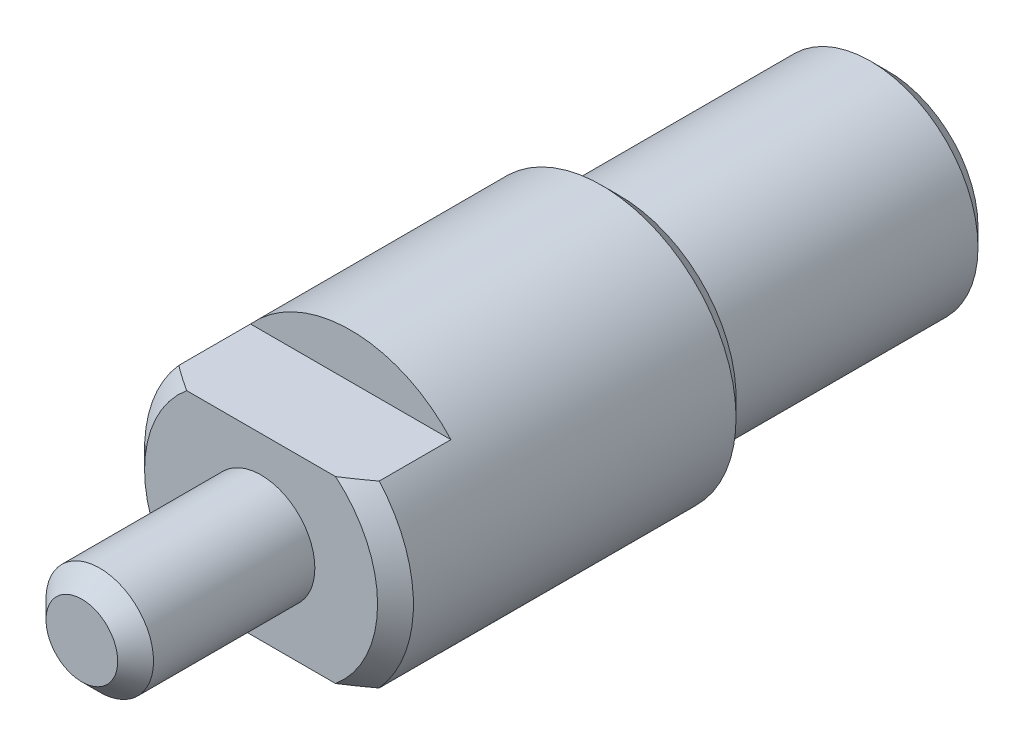
SolidWorks part; units mm, degrees
ref_plane "前视基准面" through (0, 0, 0) normal (0, 0, 1) x (1, 0, 0)
ref_plane "上视基准面" through (0, 0, 0) normal (0, 1, 0) x (1, 0, 0)
ref_plane "右视基准面" through (0, 0, 0) normal (1, 0, 0) x (0, 0, -1)
sketch "草图1" plane through (0, 0, 0) normal (0, 0, 1) x (1, 0, 0)
  circle A0 centre (0, 0) radius 7.5
  dimension "D1" = 15
extrude "凸台-拉伸1" add sketch "草图1" along normal blind 30 and the other way blind 15
sketch "草图2" plane through (0, 0, 30) normal (0, 0, 1) x (1, 0, 0)
  circle A0 centre (0, 0) radius 7.5
  circle A1 centre (0, 0) radius 3
extrude "切除-拉伸1" cut sketch "草图2" against normal blind 10
chamfer "倒角1" distance 1 angle 45 1 edges at (3, 0, 30)
sketch "草图3" plane through (0, 0, -15) normal (0, 0, -1) x (-1, 0, 0)
  circle A0 centre (0, 0) radius 7.5
  circle A1 centre (0, 0) radius 6
  dimension "D1" = 15
  dimension "D2" = 12
extrude "切除-拉伸2" cut sketch "草图3" against normal blind 15
cosmetic thread "装饰螺纹线1" parameters "D2"=10.106
chamfer "倒角2" distance 1 angle 45 1 edges at (-6, 0, -15)
chamfer "倒角3" distance 1 angle 45 1 edges at (-7.5, 0, 0)
chamfer "倒角4" distance 1 angle 45 1 edges at (7.5, 0, 20)
sketch "草图4" plane through (0, 0, 20) normal (0, 0, 1) x (1, 0, 0)
  line L0 (-14.5127, -5) -> (11.701, -5)
  line L1 (-15.4525, 5) -> (15.1632, 5)
  line L2 (-14.5127, -5) -> (-14.5127, -12.2697)
  line L3 (-14.5127, -12.2697) -> (11.701, -12.2697)
  line L4 (11.701, -12.2697) -> (11.701, -5)
  line L5 (-15.4525, 5) -> (-15.4525, 14.3397)
  line L6 (-15.4525, 14.3397) -> (15.1632, 14.3397)
  line L7 (15.1632, 14.3397) -> (15.1632, 5)
  circle A0 centre (0, 0) radius 7.5 construction
  dimension "D1" = 5
  dimension "D2" = 5
extrude "切除-拉伸3" cut sketch "草图4" against normal blind 5
